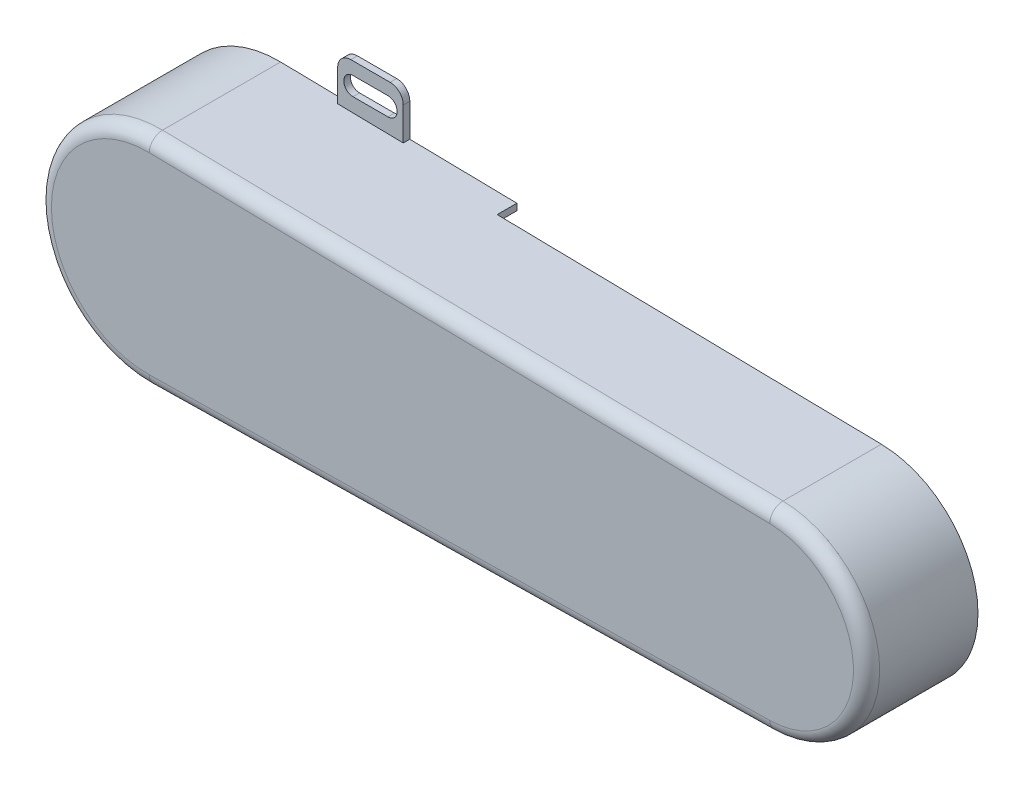
SolidWorks part; units mm, degrees
ref_plane "前视基准面" through (0, 0, 0) normal (0, 0, 1) x (1, 0, 0)
ref_plane "上视基准面" through (0, 0, 0) normal (0, 1, 0) x (1, 0, 0)
ref_plane "右视基准面" through (0, 0, 0) normal (1, 0, 0) x (0, 0, -1)
sketch "草图1" plane through (0, 0, 0) normal (0, 0, 1) x (1, 0, 0)
  line L0 (0, 0) -> (142, 0) construction
  line L1 (0.4401, 24.9961) -> (142.3961, 22.4965)
  line L2 (0.4401, -24.9961) -> (142.3961, -22.4965)
  arc A0 (0.4401, 24.9961) -> (0.4401, -24.9961) centre (0, 0) ccw
  arc A1 (142.3961, -22.4965) -> (142.3961, 22.4965) centre (142, 0) ccw
  dimension "D1" = 50
  dimension "D2" = 45
  dimension "D3" = 142
extrude "凸台-拉伸1" add sketch "草图1" along normal blind 30
shell "抽壳1" thickness 1.5
sketch "草图2" plane through (0, 0, 0) normal (0, 0, -1) x (-1, 0, 0)
  line L0 (-30, 24.4756) -> (-30, 35)
  line L1 (-142.3961, 22.4965) -> (-0.4401, 24.9961) construction
  line L2 (-30, 35) -> (-15, 35)
  line L3 (-15, 35) -> (-15, 24.7397)
  line L4 (-15, 24.7397) -> (-30, 24.4756)
  line L5 (0, 0) -> (-142, 0) construction
  dimension "D1" = 35
  dimension "D2" = 15
  dimension "D3" = 15
extrude "凸台-拉伸2" add sketch "草图2" against normal blind 1.5
sketch "草图3" plane through (0, 0, 1.5) normal (0, 0, 1) x (1, 0, 0)
  line L0 (26.5, 30) -> (18.5, 30) construction
  line L1 (26.5, 27.9) -> (18.5, 27.9)
  line L2 (26.5, 32.1) -> (18.5, 32.1)
  line L3 (22.5, 35) -> (22.5, 30) construction
  line L4 (15, 35) -> (30, 35) construction
  arc A0 (26.5, 27.9) -> (26.5, 32.1) centre (26.5, 30) ccw
  arc A1 (18.5, 32.1) -> (18.5, 27.9) centre (18.5, 30) ccw
  point P2 (22.5, 30)
  point P11 (0, 0)
  dimension "D1" = 4.2
  dimension "D2" = 8
  dimension "D3" = 5
extrude "切除-拉伸1" cut sketch "草图3" against normal up to surface (1.5 mm away) up to face at (70.5709, 0, 0)
mirror "镜向1" about plane through (0, 0, 0) normal (0, 1, 0) of "切除-拉伸1", "凸台-拉伸2"
fillet "圆角1" radius 3 12 edges at (30, 35, 0.75) (15, 35, 0.75) (30, -35, 0.75) (15, -35, 0.75) (163, 0, 28.5) (71.3917, 22.2466, 28.5) (71.3917, -22.2466, 28.5) (-23.5, 0, 28.5) (-25, 0, 30) (71.4181, -23.7463, 30) (71.4181, 23.7463, 30) (164.5, 0, 30)
sketch "草图4" plane through (0, 0, 0) normal (0, 1, 0) x (1, 0, 0)
  line L0 (30, 0) -> (142.3961, 0) construction
  line L1 (54.5, 0) -> (164.5, 0)
  line L2 (54.5, 0) -> (54.5, -4.5)
  line L3 (54.5, -4.5) -> (164.5, -4.5)
  line L4 (164.5, 0) -> (164.5, -4.5)
  line L5 (164.5, -27) -> (164.5, 0) construction
  dimension "D1" = 110
  dimension "D2" = 4.5
extrude "切除-拉伸2" cut sketch "草图4" against normal mid plane 60
